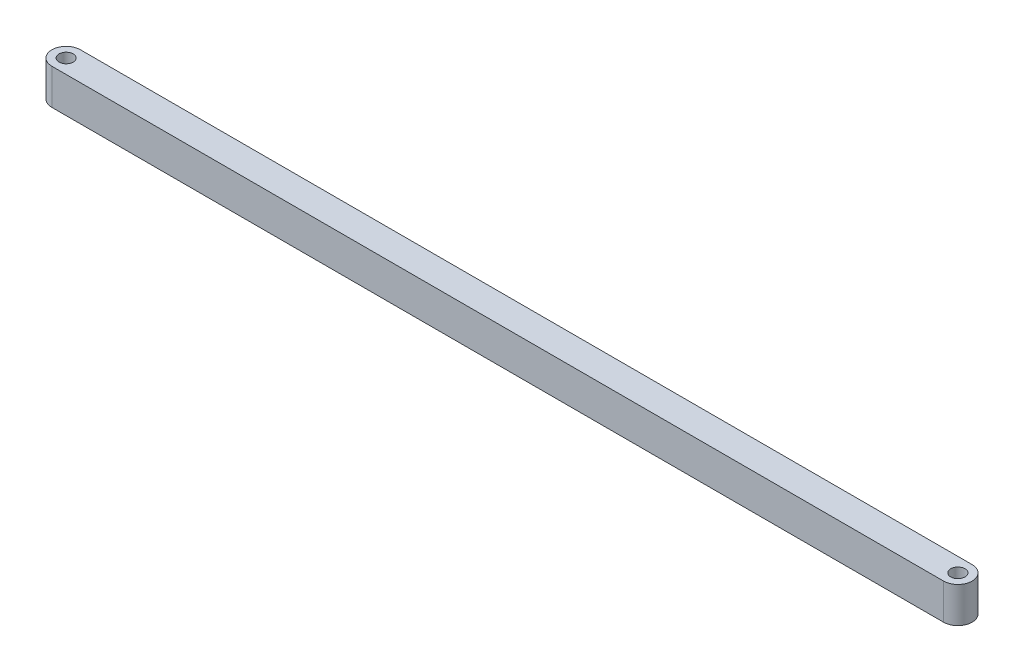
SolidWorks part; units mm, degrees
ref_plane "Front Plane" through (0, 0, 0) normal (0, 0, 1) x (1, 0, 0)
ref_plane "Top Plane" through (0, 0, 0) normal (0, 1, 0) x (1, 0, 0)
ref_plane "Right Plane" through (0, 0, 0) normal (1, 0, 0) x (0, 0, -1)
sketch "Sketch1" plane through (0, 0, 0) normal (0, 1, 0) x (1, 0, 0)
  line L0 (-125, 4) -> (125, 4)
  line L1 (125, -4) -> (-125, -4)
  line L2 (0, 34.6764) -> (0, -55.9449) construction
  arc A0 (125, 4) -> (125, -4) centre (125, 0) cw
  arc A1 (-125, -4) -> (-125, 4) centre (-125, 0) cw
  circle A2 centre (-125, 0) radius 2
  circle A3 centre (125, 0) radius 2
  dimension "D2" = 4
  dimension "D3" = 4
  dimension "D1" = 250
  dimension "D4" = 8
extrude "Boss-Extrude1" add sketch "Sketch1" along normal blind 10
